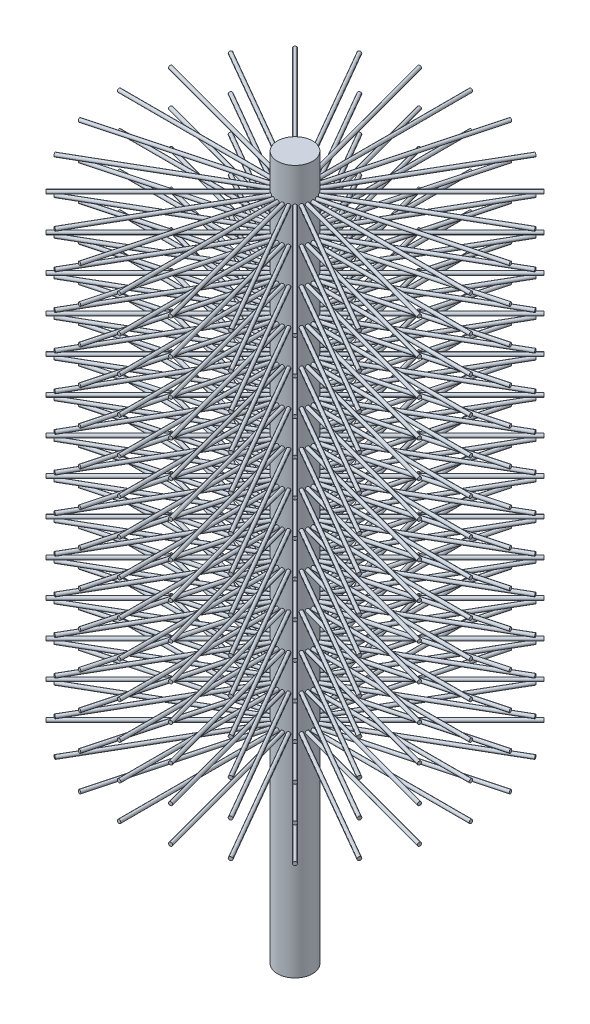
from build123d import *

# Parameters (mm, degrees)
SKETCH_1_R                = 5
EXTRUDE_1_DEPTH           = 200
SKETCH_2_R                = 0.5
EXTRUDE_2_DEPTH           = 50
PATTERN_CIRCULAR_2_COUNT  = 24
PATTERN_LINEAR_1_COUNT    = 14
PATTERN_LINEAR_1_PITCH    = 10
PATTERN_LINEAR_1_2_COUNT  = 14
PATTERN_LINEAR_1_2_PITCH  = 10
PATTERN_LINEAR_1_3_COUNT  = 14
PATTERN_LINEAR_1_3_PITCH  = 10
PATTERN_LINEAR_1_4_COUNT  = 14
PATTERN_LINEAR_1_4_PITCH  = 10
PATTERN_LINEAR_1_5_COUNT  = 14
PATTERN_LINEAR_1_5_PITCH  = 10
PATTERN_LINEAR_1_6_COUNT  = 14
PATTERN_LINEAR_1_6_PITCH  = 10
PATTERN_LINEAR_1_7_COUNT  = 14
PATTERN_LINEAR_1_7_PITCH  = 10
PATTERN_LINEAR_1_8_COUNT  = 14
PATTERN_LINEAR_1_8_PITCH  = 10
PATTERN_LINEAR_1_9_COUNT  = 14
PATTERN_LINEAR_1_9_PITCH  = 10
PATTERN_LINEAR_1_10_COUNT = 14
PATTERN_LINEAR_1_10_PITCH = 10
PATTERN_LINEAR_1_11_COUNT = 14
PATTERN_LINEAR_1_11_PITCH = 10
PATTERN_LINEAR_1_12_COUNT = 14
PATTERN_LINEAR_1_12_PITCH = 10
PATTERN_LINEAR_1_13_COUNT = 14
PATTERN_LINEAR_1_13_PITCH = 10
PATTERN_LINEAR_1_14_COUNT = 14
PATTERN_LINEAR_1_14_PITCH = 10
PATTERN_LINEAR_1_15_COUNT = 14
PATTERN_LINEAR_1_15_PITCH = 10
PATTERN_LINEAR_1_16_COUNT = 14
PATTERN_LINEAR_1_16_PITCH = 10
PATTERN_LINEAR_1_17_COUNT = 14
PATTERN_LINEAR_1_17_PITCH = 10
PATTERN_LINEAR_1_18_COUNT = 14
PATTERN_LINEAR_1_18_PITCH = 10
PATTERN_LINEAR_1_19_COUNT = 14
PATTERN_LINEAR_1_19_PITCH = 10
PATTERN_LINEAR_1_20_COUNT = 14
PATTERN_LINEAR_1_20_PITCH = 10
PATTERN_LINEAR_1_21_COUNT = 14
PATTERN_LINEAR_1_21_PITCH = 10
PATTERN_LINEAR_1_22_COUNT = 14
PATTERN_LINEAR_1_22_PITCH = 10
PATTERN_LINEAR_1_23_COUNT = 14
PATTERN_LINEAR_1_23_PITCH = 10
PATTERN_LINEAR_1_24_COUNT = 14
PATTERN_LINEAR_1_24_PITCH = 10


with BuildPart() as part:
    # 草图1 → 凸台-拉伸1 (new body)
    with BuildSketch(Plane(origin=(0, 0, 0), x_dir=(1, 0, 0), z_dir=(0, 1, 0))):
        with Locations(Location((0, 0, 0), (0, 0, 270))):
            Circle(SKETCH_1_R)
    extrude(amount=EXTRUDE_1_DEPTH)


with BuildPart() as body_2:
    # 草图2 → 凸台-拉伸2 (new body)
    with BuildSketch(Plane.XY):
        with Locations((0, 60)):
            Circle(SKETCH_2_R)
    extrude(amount=EXTRUDE_2_DEPTH)


with BuildPart() as pattern_circular_2_1:
    # 阵列(圆周)2: pattern copy
    add(body_2.part.rotate(Axis((0, 0, 0), (0, 1, 0)), 1 * 360 / PATTERN_CIRCULAR_2_COUNT))

    # Pattern Linear 1 10: 阵列(圆周)2_1 ×14


with BuildPart() as pattern_circular_2_2:
    # 阵列(圆周)2: pattern copy
    add(body_2.part.rotate(Axis((0, 0, 0), (0, 1, 0)), 2 * 360 / PATTERN_CIRCULAR_2_COUNT))

    # Pattern Linear 1 20: 阵列(圆周)2_2 ×14


with BuildPart() as pattern_circular_2_3:
    # 阵列(圆周)2: pattern copy
    add(body_2.part.rotate(Axis((0, 0, 0), (0, 1, 0)), 3 * 360 / PATTERN_CIRCULAR_2_COUNT))

    # Pattern Linear 1 6: 阵列(圆周)2_3 ×14


with BuildPart() as pattern_circular_2_4:
    # 阵列(圆周)2: pattern copy
    add(body_2.part.rotate(Axis((0, 0, 0), (0, 1, 0)), 4 * 360 / PATTERN_CIRCULAR_2_COUNT))

    # Pattern Linear 1 17: 阵列(圆周)2_4 ×14


with BuildPart() as pattern_circular_2_5:
    # 阵列(圆周)2: pattern copy
    add(body_2.part.rotate(Axis((0, 0, 0), (0, 1, 0)), 5 * 360 / PATTERN_CIRCULAR_2_COUNT))

    # Pattern Linear 1 3: 阵列(圆周)2_5 ×14


with BuildPart() as pattern_circular_2_6:
    # 阵列(圆周)2: pattern copy
    add(body_2.part.rotate(Axis((0, 0, 0), (0, 1, 0)), 6 * 360 / PATTERN_CIRCULAR_2_COUNT))

    # Pattern Linear 1 15: 阵列(圆周)2_6 ×14


with BuildPart() as pattern_circular_2_7:
    # 阵列(圆周)2: pattern copy
    add(body_2.part.rotate(Axis((0, 0, 0), (0, 1, 0)), 7 * 360 / PATTERN_CIRCULAR_2_COUNT))

    # 阵列(线性)1: 阵列(圆周)2_7 ×14


with BuildPart() as pattern_circular_2_8:
    # 阵列(圆周)2: pattern copy
    add(body_2.part.rotate(Axis((0, 0, 0), (0, 1, 0)), 8 * 360 / PATTERN_CIRCULAR_2_COUNT))

    # Pattern Linear 1 13: 阵列(圆周)2_8 ×14


with BuildPart() as pattern_circular_2_9:
    # 阵列(圆周)2: pattern copy
    add(body_2.part.rotate(Axis((0, 0, 0), (0, 1, 0)), 9 * 360 / PATTERN_CIRCULAR_2_COUNT))

    # Pattern Linear 1 23: 阵列(圆周)2_9 ×14


with BuildPart() as pattern_circular_2_10:
    # 阵列(圆周)2: pattern copy
    add(body_2.part.rotate(Axis((0, 0, 0), (0, 1, 0)), 10 * 360 / PATTERN_CIRCULAR_2_COUNT))

    # Pattern Linear 1 11: 阵列(圆周)2_10 ×14


with BuildPart() as pattern_circular_2_11:
    # 阵列(圆周)2: pattern copy
    add(body_2.part.rotate(Axis((0, 0, 0), (0, 1, 0)), 11 * 360 / PATTERN_CIRCULAR_2_COUNT))

    # Pattern Linear 1 21: 阵列(圆周)2_11 ×14


with BuildPart() as pattern_circular_2_12:
    # 阵列(圆周)2: pattern copy
    add(body_2.part.rotate(Axis((0, 0, 0), (0, 1, 0)), 12 * 360 / PATTERN_CIRCULAR_2_COUNT))

    # Pattern Linear 1 7: 阵列(圆周)2_12 ×14


with BuildPart() as pattern_circular_2_13:
    # 阵列(圆周)2: pattern copy
    add(body_2.part.rotate(Axis((0, 0, 0), (0, 1, 0)), 13 * 360 / PATTERN_CIRCULAR_2_COUNT))

    # Pattern Linear 1 18: 阵列(圆周)2_13 ×14


with BuildPart() as pattern_circular_2_14:
    # 阵列(圆周)2: pattern copy
    add(body_2.part.rotate(Axis((0, 0, 0), (0, 1, 0)), 14 * 360 / PATTERN_CIRCULAR_2_COUNT))

    # Pattern Linear 1 4: 阵列(圆周)2_14 ×14


with BuildPart() as pattern_circular_2_15:
    # 阵列(圆周)2: pattern copy
    add(body_2.part.rotate(Axis((0, 0, 0), (0, 1, 0)), 15 * 360 / PATTERN_CIRCULAR_2_COUNT))

    # Pattern Linear 1 16: 阵列(圆周)2_15 ×14


with BuildPart() as pattern_circular_2_16:
    # 阵列(圆周)2: pattern copy
    add(body_2.part.rotate(Axis((0, 0, 0), (0, 1, 0)), 16 * 360 / PATTERN_CIRCULAR_2_COUNT))

    # Pattern Linear 1 2: 阵列(圆周)2_16 ×14


with BuildPart() as pattern_circular_2_17:
    # 阵列(圆周)2: pattern copy
    add(body_2.part.rotate(Axis((0, 0, 0), (0, 1, 0)), 17 * 360 / PATTERN_CIRCULAR_2_COUNT))

    # Pattern Linear 1 14: 阵列(圆周)2_17 ×14


with BuildPart() as pattern_circular_2_18:
    # 阵列(圆周)2: pattern copy
    add(body_2.part.rotate(Axis((0, 0, 0), (0, 1, 0)), 18 * 360 / PATTERN_CIRCULAR_2_COUNT))

    # Pattern Linear 1 24: 阵列(圆周)2_18 ×14


with BuildPart() as pattern_circular_2_19:
    # 阵列(圆周)2: pattern copy
    add(body_2.part.rotate(Axis((0, 0, 0), (0, 1, 0)), 19 * 360 / PATTERN_CIRCULAR_2_COUNT))

    # Pattern Linear 1 12: 阵列(圆周)2_19 ×14


with BuildPart() as pattern_circular_2_20:
    # 阵列(圆周)2: pattern copy
    add(body_2.part.rotate(Axis((0, 0, 0), (0, 1, 0)), 20 * 360 / PATTERN_CIRCULAR_2_COUNT))

    # Pattern Linear 1 22: 阵列(圆周)2_20 ×14


with BuildPart() as pattern_circular_2_21:
    # 阵列(圆周)2: pattern copy
    add(body_2.part.rotate(Axis((0, 0, 0), (0, 1, 0)), 21 * 360 / PATTERN_CIRCULAR_2_COUNT))

    # Pattern Linear 1 8: 阵列(圆周)2_21 ×14


with BuildPart() as pattern_circular_2_22:
    # 阵列(圆周)2: pattern copy
    add(body_2.part.rotate(Axis((0, 0, 0), (0, 1, 0)), 22 * 360 / PATTERN_CIRCULAR_2_COUNT))

    # Pattern Linear 1 19: 阵列(圆周)2_22 ×14


with BuildPart() as pattern_circular_2_23:
    # 阵列(圆周)2: pattern copy
    add(body_2.part.rotate(Axis((0, 0, 0), (0, 1, 0)), 23 * 360 / PATTERN_CIRCULAR_2_COUNT))

    # Pattern Linear 1 5: 阵列(圆周)2_23 ×14


with BuildPart() as pattern_circular_2_7_1:
    add(pattern_circular_2_7.part)
    with Locations(*[(0, i * PATTERN_LINEAR_1_PITCH, 0) for i in range(1, PATTERN_LINEAR_1_COUNT)]):
        add(pattern_circular_2_7.part)


with BuildPart() as pattern_circular_2_16_1:
    add(pattern_circular_2_16.part)
    with Locations(*[(0, i * PATTERN_LINEAR_1_2_PITCH, 0) for i in range(1, PATTERN_LINEAR_1_2_COUNT)]):
        add(pattern_circular_2_16.part)


with BuildPart() as pattern_circular_2_5_1:
    add(pattern_circular_2_5.part)
    with Locations(*[(0, i * PATTERN_LINEAR_1_3_PITCH, 0) for i in range(1, PATTERN_LINEAR_1_3_COUNT)]):
        add(pattern_circular_2_5.part)


with BuildPart() as pattern_circular_2_14_1:
    add(pattern_circular_2_14.part)
    with Locations(*[(0, i * PATTERN_LINEAR_1_4_PITCH, 0) for i in range(1, PATTERN_LINEAR_1_4_COUNT)]):
        add(pattern_circular_2_14.part)


with BuildPart() as pattern_circular_2_23_1:
    add(pattern_circular_2_23.part)
    with Locations(*[(0, i * PATTERN_LINEAR_1_5_PITCH, 0) for i in range(1, PATTERN_LINEAR_1_5_COUNT)]):
        add(pattern_circular_2_23.part)


with BuildPart() as pattern_circular_2_3_1:
    add(pattern_circular_2_3.part)
    with Locations(*[(0, i * PATTERN_LINEAR_1_6_PITCH, 0) for i in range(1, PATTERN_LINEAR_1_6_COUNT)]):
        add(pattern_circular_2_3.part)


with BuildPart() as pattern_circular_2_12_1:
    add(pattern_circular_2_12.part)
    with Locations(*[(0, i * PATTERN_LINEAR_1_7_PITCH, 0) for i in range(1, PATTERN_LINEAR_1_7_COUNT)]):
        add(pattern_circular_2_12.part)


with BuildPart() as pattern_circular_2_21_1:
    add(pattern_circular_2_21.part)
    with Locations(*[(0, i * PATTERN_LINEAR_1_8_PITCH, 0) for i in range(1, PATTERN_LINEAR_1_8_COUNT)]):
        add(pattern_circular_2_21.part)


with BuildPart() as body_2_1:
    add(body_2.part)

    # Pattern Linear 1 9: body 2 ×14
    with Locations(*[(0, i * PATTERN_LINEAR_1_9_PITCH, 0) for i in range(1, PATTERN_LINEAR_1_9_COUNT)]):
        add(body_2.part)


with BuildPart() as pattern_circular_2_1_1:
    add(pattern_circular_2_1.part)
    with Locations(*[(0, i * PATTERN_LINEAR_1_10_PITCH, 0) for i in range(1, PATTERN_LINEAR_1_10_COUNT)]):
        add(pattern_circular_2_1.part)


with BuildPart() as pattern_circular_2_10_1:
    add(pattern_circular_2_10.part)
    with Locations(*[(0, i * PATTERN_LINEAR_1_11_PITCH, 0) for i in range(1, PATTERN_LINEAR_1_11_COUNT)]):
        add(pattern_circular_2_10.part)


with BuildPart() as pattern_circular_2_19_1:
    add(pattern_circular_2_19.part)
    with Locations(*[(0, i * PATTERN_LINEAR_1_12_PITCH, 0) for i in range(1, PATTERN_LINEAR_1_12_COUNT)]):
        add(pattern_circular_2_19.part)


with BuildPart() as pattern_circular_2_8_1:
    add(pattern_circular_2_8.part)
    with Locations(*[(0, i * PATTERN_LINEAR_1_13_PITCH, 0) for i in range(1, PATTERN_LINEAR_1_13_COUNT)]):
        add(pattern_circular_2_8.part)


with BuildPart() as pattern_circular_2_17_1:
    add(pattern_circular_2_17.part)
    with Locations(*[(0, i * PATTERN_LINEAR_1_14_PITCH, 0) for i in range(1, PATTERN_LINEAR_1_14_COUNT)]):
        add(pattern_circular_2_17.part)


with BuildPart() as pattern_circular_2_6_1:
    add(pattern_circular_2_6.part)
    with Locations(*[(0, i * PATTERN_LINEAR_1_15_PITCH, 0) for i in range(1, PATTERN_LINEAR_1_15_COUNT)]):
        add(pattern_circular_2_6.part)


with BuildPart() as pattern_circular_2_15_1:
    add(pattern_circular_2_15.part)
    with Locations(*[(0, i * PATTERN_LINEAR_1_16_PITCH, 0) for i in range(1, PATTERN_LINEAR_1_16_COUNT)]):
        add(pattern_circular_2_15.part)


with BuildPart() as pattern_circular_2_4_1:
    add(pattern_circular_2_4.part)
    with Locations(*[(0, i * PATTERN_LINEAR_1_17_PITCH, 0) for i in range(1, PATTERN_LINEAR_1_17_COUNT)]):
        add(pattern_circular_2_4.part)


with BuildPart() as pattern_circular_2_13_1:
    add(pattern_circular_2_13.part)
    with Locations(*[(0, i * PATTERN_LINEAR_1_18_PITCH, 0) for i in range(1, PATTERN_LINEAR_1_18_COUNT)]):
        add(pattern_circular_2_13.part)


with BuildPart() as pattern_circular_2_22_1:
    add(pattern_circular_2_22.part)
    with Locations(*[(0, i * PATTERN_LINEAR_1_19_PITCH, 0) for i in range(1, PATTERN_LINEAR_1_19_COUNT)]):
        add(pattern_circular_2_22.part)


with BuildPart() as pattern_circular_2_2_1:
    add(pattern_circular_2_2.part)
    with Locations(*[(0, i * PATTERN_LINEAR_1_20_PITCH, 0) for i in range(1, PATTERN_LINEAR_1_20_COUNT)]):
        add(pattern_circular_2_2.part)


with BuildPart() as pattern_circular_2_11_1:
    add(pattern_circular_2_11.part)
    with Locations(*[(0, i * PATTERN_LINEAR_1_21_PITCH, 0) for i in range(1, PATTERN_LINEAR_1_21_COUNT)]):
        add(pattern_circular_2_11.part)


with BuildPart() as pattern_circular_2_20_1:
    add(pattern_circular_2_20.part)
    with Locations(*[(0, i * PATTERN_LINEAR_1_22_PITCH, 0) for i in range(1, PATTERN_LINEAR_1_22_COUNT)]):
        add(pattern_circular_2_20.part)


with BuildPart() as pattern_circular_2_9_1:
    add(pattern_circular_2_9.part)
    with Locations(*[(0, i * PATTERN_LINEAR_1_23_PITCH, 0) for i in range(1, PATTERN_LINEAR_1_23_COUNT)]):
        add(pattern_circular_2_9.part)


with BuildPart() as pattern_circular_2_18_1:
    add(pattern_circular_2_18.part)
    with Locations(*[(0, i * PATTERN_LINEAR_1_24_PITCH, 0) for i in range(1, PATTERN_LINEAR_1_24_COUNT)]):
        add(pattern_circular_2_18.part)


solid = Compound([part.part, pattern_circular_2_7_1.part, pattern_circular_2_16_1.part, pattern_circular_2_5_1.part, pattern_circular_2_14_1.part, pattern_circular_2_23_1.part, pattern_circular_2_3_1.part, pattern_circular_2_12_1.part, pattern_circular_2_21_1.part, body_2_1.part, pattern_circular_2_1_1.part, pattern_circular_2_10_1.part, pattern_circular_2_19_1.part, pattern_circular_2_8_1.part, pattern_circular_2_17_1.part, pattern_circular_2_6_1.part, pattern_circular_2_15_1.part, pattern_circular_2_4_1.part, pattern_circular_2_13_1.part, pattern_circular_2_22_1.part, pattern_circular_2_2_1.part, pattern_circular_2_11_1.part, pattern_circular_2_20_1.part, pattern_circular_2_9_1.part, pattern_circular_2_18_1.part])
